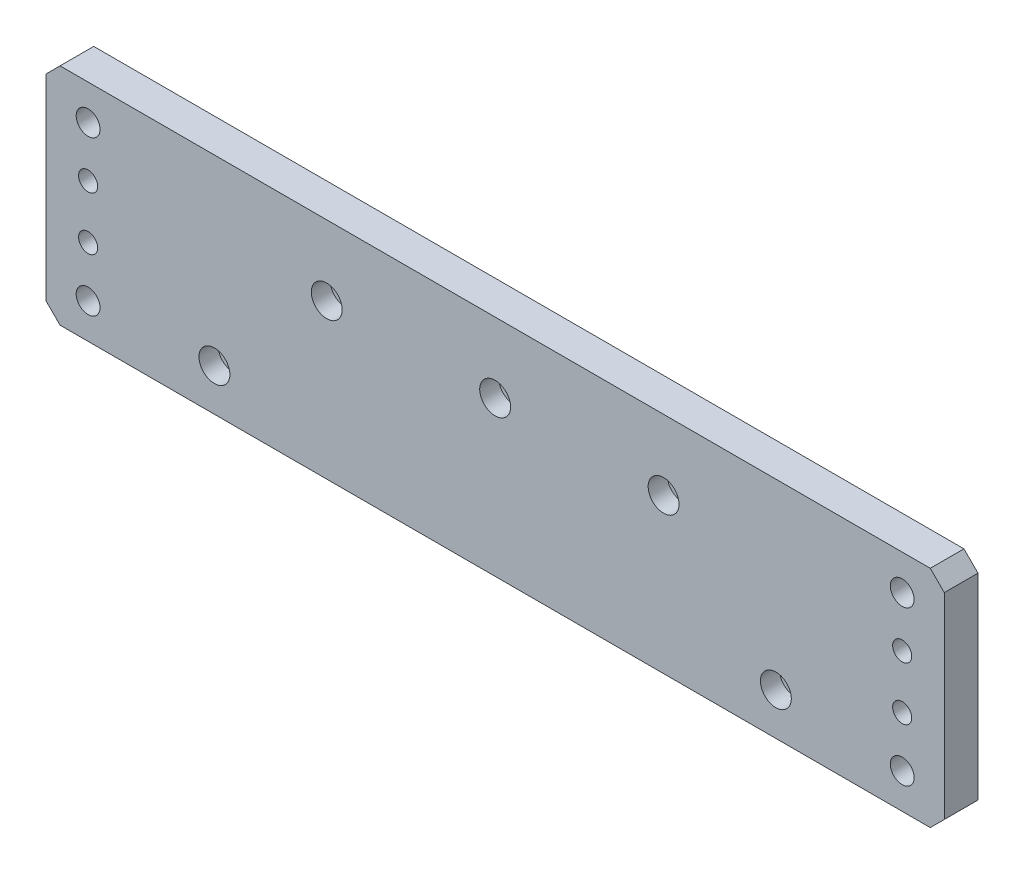
from build123d import *

# Parameters (mm, degrees)
SKETCH_1_W                = 320
SKETCH_1_H                = 80
EXTRUDE_1_DEPTH           = 12
CHAMFER_1_SIZE            = 5
HOLE_WIZARD_M8_1_D        = 6.8
HOLE_WIZARD_8_5_8_5_1_D   = 8.5
HOLE_WIZARD_1_D           = 6.6
HOLE_WIZARD_1_CBORE_D     = 11
HOLE_WIZARD_1_CBORE_DEPTH = 6.8


with BuildPart() as part:
    # 草图1 → 凸台-拉伸1 (new body)
    with BuildSketch(Plane.XY):
        Rectangle(SKETCH_1_W, SKETCH_1_H)
    extrude(amount=EXTRUDE_1_DEPTH)

    # 倒角1
    chamfer_1_edges = [part.edges().sort_by_distance(p)[0] for p in [
        (160, -40, 6),
        (-160, -40, 6),
        (-160, 40, 6),
        (160, 40, 6),
    ]]
    chamfer(chamfer_1_edges, length=CHAMFER_1_SIZE)

    # M8 螺纹孔1 (through all)
    with Locations(Plane(origin=(0, 0, 0), x_dir=(-1, 0, 0), z_dir=(0, 0, -1))):
        with Locations((-145, 9.5), (-145, -9.5), (145, 9.5), (145, -9.5)):
            Hole(HOLE_WIZARD_M8_1_D / 2)

    # Ø8.5 (8.5) 直径孔1 (through all)
    with Locations(Plane(origin=(0, 0, 0), x_dir=(-1, 0, 0), z_dir=(0, 0, -1))):
        with Locations((-145, 27.5), (-145, -27.5), (145, 27.5), (145, -27.5)):
            Hole(HOLE_WIZARD_8_5_8_5_1_D / 2)

    # 打孔尺寸(%根据)内六角圆柱头螺钉的类型1 (through all)
    with Locations(Plane.XY.offset(12)):
        with Locations((-60, 15), (0, 15), (60, 15), (100, -25), (-100, -25)):
            CounterBoreHole(HOLE_WIZARD_1_D / 2, HOLE_WIZARD_1_CBORE_D / 2, HOLE_WIZARD_1_CBORE_DEPTH)


solid = part.part
